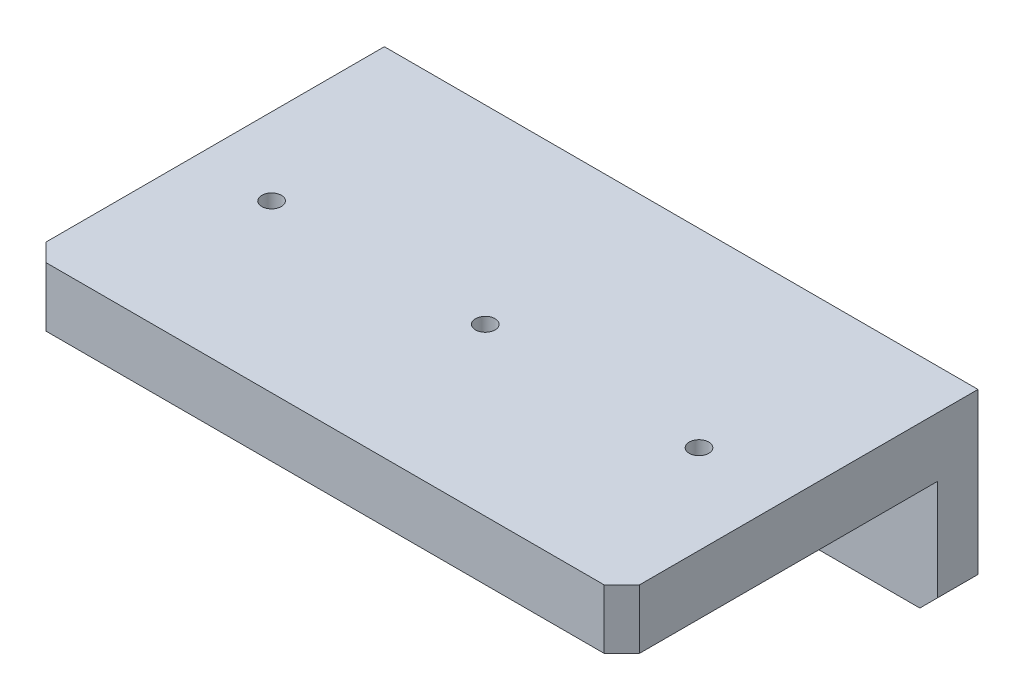
from build123d import *

# Parameters (mm, degrees)
SKETCH_1_W                = 100
SKETCH_1_H                = 60
EXTRUDE_1_DEPTH           = 10
SKETCH_2_W                = 100
SKETCH_2_H                = 6.8
EXTRUDE_2_DEPTH           = 20
CHAMFER_1_SIZE            = 3
HOLE_WIZARD_M4_1_D        = 3.3
HOLE_WIZARD_M4_1_DEPTH    = 10.1
HOLE_WIZARD_M4_1_TIP      = 0.991420021
HOLE_WIZARD_1_D           = 5.5
HOLE_WIZARD_1_DEPTH       = 10.1
HOLE_WIZARD_1_CSINK_D     = 11.2
HOLE_WIZARD_1_CSINK_ANGLE = 90
HOLE_WIZARD_1_TIP         = 1.652366702


with BuildPart() as part:
    # 草图1 → 凸台-拉伸1 (new body)
    with BuildSketch(Plane(origin=(0, 0, 0), x_dir=(1, 0, 0), z_dir=(0, 1, 0))):
        Rectangle(SKETCH_1_W, SKETCH_1_H)
    extrude(amount=EXTRUDE_1_DEPTH)

    # 草图2 → 凸台-拉伸2 (add)
    with BuildSketch(Plane.XZ):
        with Locations((0, -26.6)):
            Rectangle(SKETCH_2_W, SKETCH_2_H)
    extrude(amount=EXTRUDE_2_DEPTH)

    # 倒角1
    chamfer_1_edges = [part.edges().sort_by_distance(p)[0] for p in [
        (50, -20, -26.6),
        (-50, -20, -26.6),
        (50, 5, 30),
        (-50, 5, 30),
    ]]
    chamfer(chamfer_1_edges, length=CHAMFER_1_SIZE)

    # M4 螺纹孔1
    with Locations(Plane(origin=(0, 10, 0), x_dir=(1, 0, 0), z_dir=(0, 1, 0))):
        with Locations((35, -2), (-37, -2), (-1, -2)):
            Hole(HOLE_WIZARD_M4_1_D / 2, depth=HOLE_WIZARD_M4_1_DEPTH)
            with Locations((0, 0, -(HOLE_WIZARD_M4_1_DEPTH + HOLE_WIZARD_M4_1_TIP / 2))):  # 118° drill point
                Cone(0, HOLE_WIZARD_M4_1_D / 2, HOLE_WIZARD_M4_1_TIP, mode=Mode.SUBTRACT)

    # 打孔尺寸(%根据)开槽半沉头木螺钉的类型1
    with Locations(Plane.XY.offset(-23.2)):
        with Locations((-10, -10), (-25, -10)):
            CounterSinkHole(HOLE_WIZARD_1_D / 2, HOLE_WIZARD_1_CSINK_D / 2, depth=HOLE_WIZARD_1_DEPTH, counter_sink_angle=HOLE_WIZARD_1_CSINK_ANGLE)
            with Locations((0, 0, -(HOLE_WIZARD_1_DEPTH + HOLE_WIZARD_1_TIP / 2))):  # 118° drill point
                Cone(0, HOLE_WIZARD_1_D / 2, HOLE_WIZARD_1_TIP, mode=Mode.SUBTRACT)


solid = part.part
